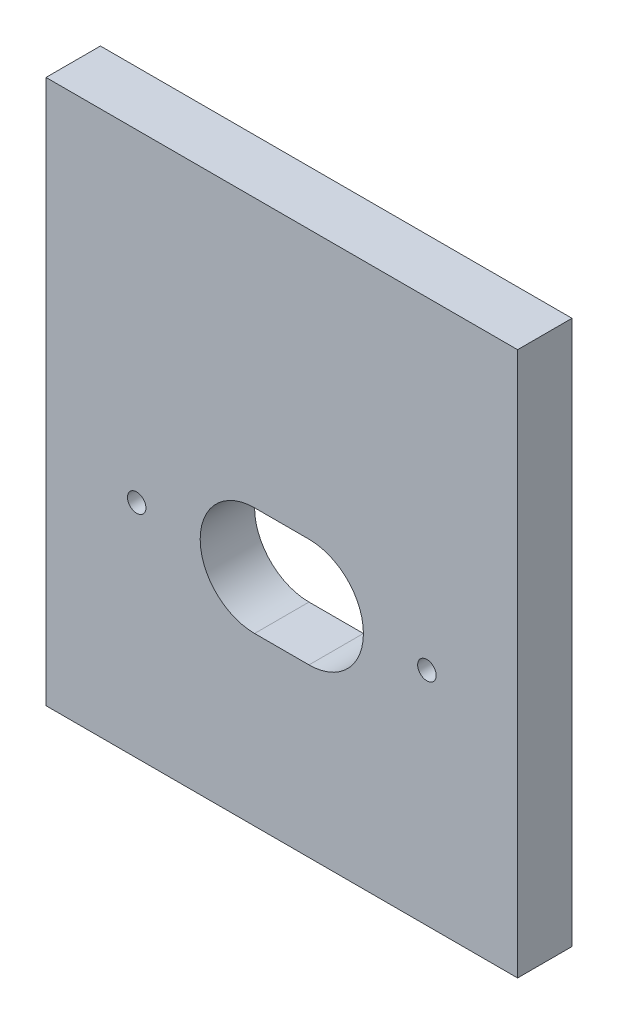
SolidWorks part; units mm, degrees
material "Q235"
ref_plane "Front Plane" through (0, 0, 0) normal (0, 0, 1) x (1, 0, 0)
ref_plane "Top Plane" through (0, 0, 0) normal (0, 1, 0) x (1, 0, 0)
ref_plane "Right Plane" through (0, 0, 0) normal (1, 0, 0) x (0, 0, -1)
sketch "Sketch1" plane through (0, 0, 0) normal (0, 0, 1) x (1, 0, 0)
  line L0 (130, 300) -> (130, 0) construction
  line L1 (0, 0) -> (260, 0)
  line L2 (0, 0) -> (0, 300)
  line L3 (0, 300) -> (260, 300)
  line L4 (260, 0) -> (260, 300)
  line L5 (0, 122) -> (260, 122) construction
  line L6 (115, 122) -> (145, 122) construction
  line L7 (115, 152) -> (145, 152)
  line L8 (115, 92) -> (145, 92)
  arc A0 (115, 152) -> (115, 92) centre (115, 122) ccw
  arc A1 (145, 92) -> (145, 152) centre (145, 122) ccw
  point P11 (130, 122)
  dimension "D5" = 30
  dimension "D1" = 300
  dimension "D2" = 260
  dimension "D3" = 178
  dimension "D4" = 30
extrude "Boss-Extrude1" add sketch "Sketch1" along normal blind 30
hole_wizard "M12 Threaded hole1" positions "3DSketch1" profile "Sketch2" tap size "M12" standard "GB" end condition through all
sketch3d "3DSketch1"
  line L0 (260, 300, 30) -> (0, 300, 30) construction
  point P0 (50, 122, 30)
  point P2 (210, 122, 30)
  dimension "D1" = 178
  dimension "D2" = 178
  dimension "D3" = 160
  dimension "D4" = 50
sketch "Sketch2" plane through (50, 122, 30) normal (1, 0, 0) x (0, -1, 0)
  line L0 (0, 0) -> (0, 30)
  line L1 (0, 30) -> (5.1, 30)
  line L2 (5.1, 30) -> (5.1, 0)
  line L5 (5.1, 0) -> (0, 0)
  line L11 (0, -6.35) -> (0, 107.95) construction
  dimension "通孔螺纹孔钻头直径" = 10.2
  dimension "通孔螺纹孔钻头深度" = 30
cosmetic thread "孔螺蚊线1" parameters "D2"=12
cosmetic thread "孔螺蚊线2" parameters "D2"=12
